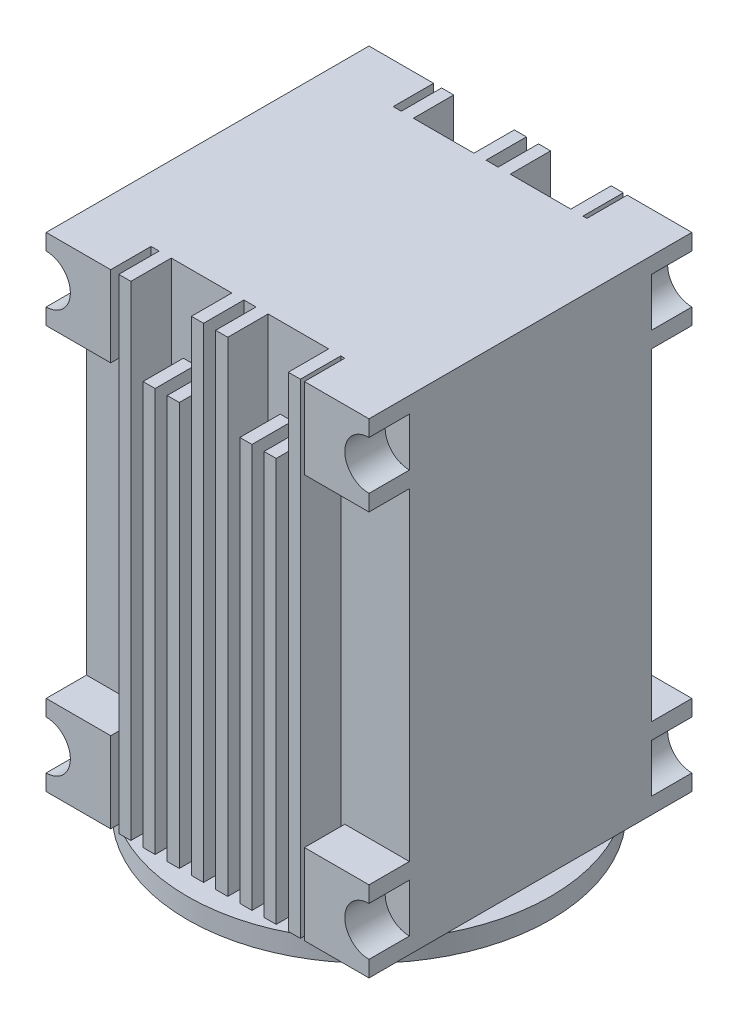
from build123d import *

# Parameters (mm, degrees)
SKETCH1_W           = 40
SKETCH1_H           = 40
BOSS_EXTRUDE1_DEPTH = 30
CUT_EXTRUDE1_DEPTH  = 5
SKETCH3_W           = 1.5
SKETCH3_H           = 5
BOSS_EXTRUDE2_DEPTH = 60
SKETCH4_W           = 4.5
SKETCH4_H           = 10
CUT_EXTRUDE2_DEPTH  = 5
SKETCH5_R           = 3
CUT_EXTRUDE3_DEPTH  = 5
SKETCH6_R           = 22.5
BOSS_EXTRUDE3_DEPTH = 2.5
SKETCH7_R           = 5
CUT_EXTRUDE4_DEPTH  = 15
SKETCH8_R           = 2.5
CUT_EXTRUDE5_DEPTH  = 10
SKETCH9_R           = 1
CUT_EXTRUDE6_DEPTH  = 1.8


with BuildPart() as part:
    # Sketch1 → Boss-Extrude1 (new, symmetric)
    with BuildSketch(Plane(origin=(0, 0, 0), x_dir=(1, 0, 0), z_dir=(0, 1, 0))):
        Rectangle(SKETCH1_W, SKETCH1_H)
    extrude(amount=BOSS_EXTRUDE1_DEPTH, both=True)

    # Sketch2 → Cut-Extrude1 (cut)
    with BuildSketch(Plane(origin=(0, 0, -20), x_dir=(-1, 0, 0), z_dir=(0, 0, -1))):
        Polygon((-12, 30), (12, 30), (12, 20), (20, 20), (20, -20), (12, -20), (12, -30), (-12, -30), (-12, -20), (-20, -20), (-20, 20), (-12, 20), align=None)
    cut_extrude1 = extrude(amount=-CUT_EXTRUDE1_DEPTH, mode=Mode.SUBTRACT)

    # Mirror1: Cut-Extrude1 across plane
    add(cut_extrude1.mirror(Plane.XY), mode=Mode.SUBTRACT)

    # Sketch3 → Boss-Extrude2 (add)
    with BuildSketch(Plane(origin=(0, 30, 0), x_dir=(1, 0, 0), z_dir=(0, 1, 0))):
        with Locations((-10.25, 17.5)):
            Rectangle(SKETCH3_W, SKETCH3_H)
        with Locations((-7.25, 17.5)):
            Rectangle(SKETCH3_W, SKETCH3_H)
        with Locations((-4.25, 17.5)):
            Rectangle(SKETCH3_W, SKETCH3_H)
        with Locations((-1.25, 17.5)):
            Rectangle(SKETCH3_W, SKETCH3_H)
        with Locations((1.75, 17.5)):
            Rectangle(SKETCH3_W, SKETCH3_H)
        with Locations((4.75, 17.5)):
            Rectangle(SKETCH3_W, SKETCH3_H)
        with Locations((7.75, 17.5)):
            Rectangle(SKETCH3_W, SKETCH3_H)
        with Locations((10.75, 17.5)):
            Rectangle(SKETCH3_W, SKETCH3_H)
    boss_extrude2 = extrude(amount=-BOSS_EXTRUDE2_DEPTH)

    # Sketch4 → Cut-Extrude2 (cut)
    with BuildSketch(Plane(origin=(0, 0, -20), x_dir=(-1, 0, 0), z_dir=(0, 0, -1))):
        with Locations((-6.25, 25)):
            Rectangle(SKETCH4_W, SKETCH4_H)
        with Locations((5.75, 25)):
            Rectangle(SKETCH4_W, SKETCH4_H)
    cut_extrude2 = extrude(amount=-CUT_EXTRUDE2_DEPTH, mode=Mode.SUBTRACT)

    # Mirror2: Boss-Extrude2, Cut-Extrude2 across plane
    add(boss_extrude2.mirror(Plane.XY))
    add(cut_extrude2.mirror(Plane.XY), mode=Mode.SUBTRACT)

    # Sketch5 → Cut-Extrude3 (cut)
    with BuildSketch(Plane(origin=(0, 0, -20), x_dir=(-1, 0, 0), z_dir=(0, 0, -1))):
        with Locations((-20, 25)):
            Circle(SKETCH5_R)
        with Locations((20, 25)):
            Circle(SKETCH5_R)
        with Locations((-20, -25)):
            Circle(SKETCH5_R)
        with Locations((20, -25)):
            Circle(SKETCH5_R)
    cut_extrude3 = extrude(amount=-CUT_EXTRUDE3_DEPTH, mode=Mode.SUBTRACT)

    # Mirror3: Cut-Extrude3 across plane
    add(cut_extrude3.mirror(Plane.XY), mode=Mode.SUBTRACT)

    # Sketch6 → Boss-Extrude3 (add)
    with BuildSketch(Plane.XZ.offset(30)):
        with Locations(Location((0, 0, 0), (0, 0, 62.733955549))):
            Circle(SKETCH6_R)
    extrude(amount=BOSS_EXTRUDE3_DEPTH)

    # Sketch7 → Cut-Extrude4 (cut)
    with BuildSketch(Plane.XZ.offset(32.5)):
        with Locations(Location((0, 0, 0), (0, 0, 270))):
            Circle(SKETCH7_R)
    extrude(amount=-CUT_EXTRUDE4_DEPTH, mode=Mode.SUBTRACT)

    # Sketch8 → Cut-Extrude5 (cut)
    with BuildSketch(Plane.ZY.offset(20)):
        with Locations((-0.51, 13.59)):
            Circle(SKETCH8_R)
    extrude(amount=-CUT_EXTRUDE5_DEPTH, mode=Mode.SUBTRACT)

    # Sketch9 → Cut-Extrude6 (cut)
    with BuildSketch(Plane.XZ.offset(30)):
        with Locations(Location((-17.5, 17.5, 0), (0, 0, 270))):
            Circle(SKETCH9_R)
        with Locations(Location((17.5, 17.5, 0), (0, 0, 270))):
            Circle(SKETCH9_R)
        with Locations(Location((17.5, -17.5, 0), (0, 0, 270))):
            Circle(SKETCH9_R)
        with Locations(Location((-17.5, -17.5, 0), (0, 0, 270))):
            Circle(SKETCH9_R)
    extrude(amount=-CUT_EXTRUDE6_DEPTH, mode=Mode.SUBTRACT)


solid = part.part
